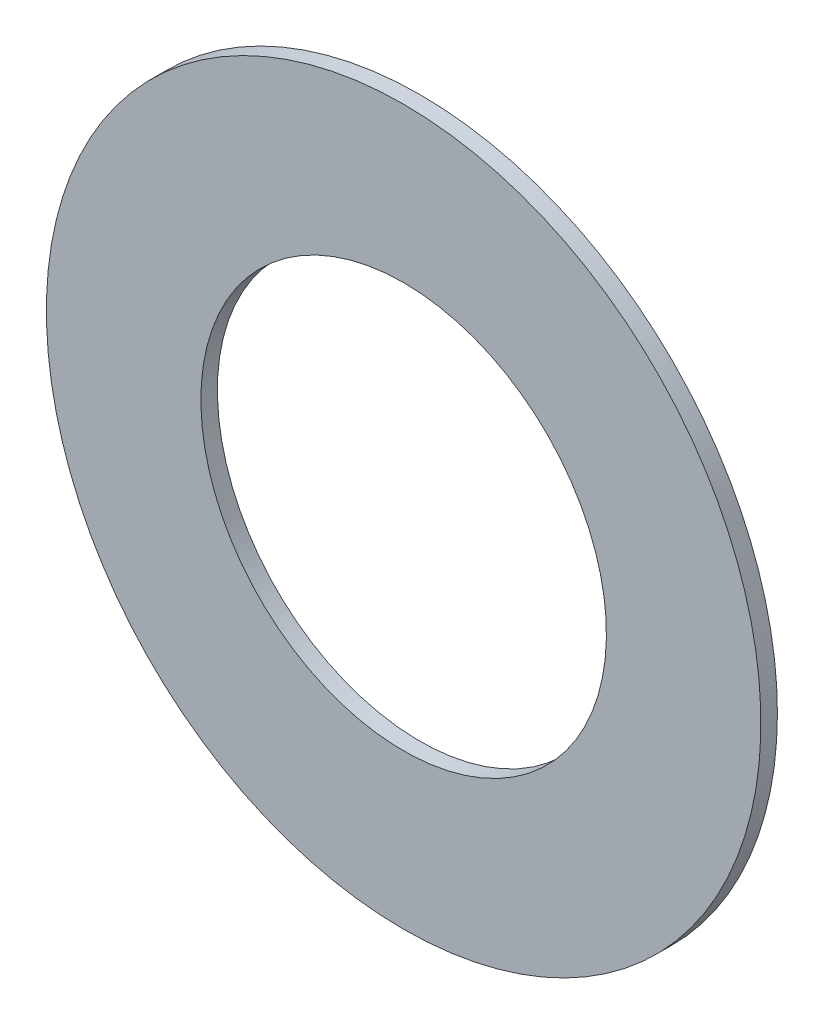
from build123d import *

# Parameters (mm, degrees)
SKETCH1_R           = 37
SKETCH1_R_2         = 21
BOSS_EXTRUDE1_DEPTH = 1.71


with BuildPart() as part:
    # Sketch1 → Boss-Extrude1 (new body)
    with BuildSketch(Plane.XY):
        with Locations(Location((0, 0, 0), (0, 0, 90))):
            Circle(SKETCH1_R)
        with Locations(Location((0, 0, 0), (0, 0, 90))):
            Circle(SKETCH1_R_2, mode=Mode.SUBTRACT)
    extrude(amount=BOSS_EXTRUDE1_DEPTH)


solid = part.part
